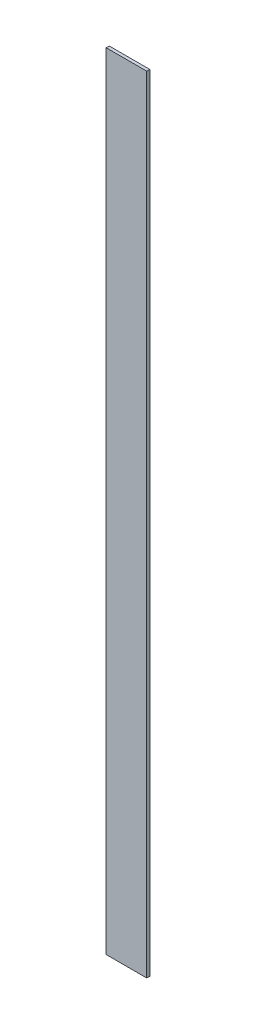
from build123d import *

# Parameters (mm, degrees)
SKETCH1_W           = 400
SKETCH1_H           = 7756
BOSS_EXTRUDE1_DEPTH = 15


with BuildPart() as part:
    # Sketch1 → Boss-Extrude1 (new, symmetric)
    with BuildSketch(Plane.XY):
        Rectangle(SKETCH1_W, SKETCH1_H)
    extrude(amount=BOSS_EXTRUDE1_DEPTH, both=True)


solid = part.part
